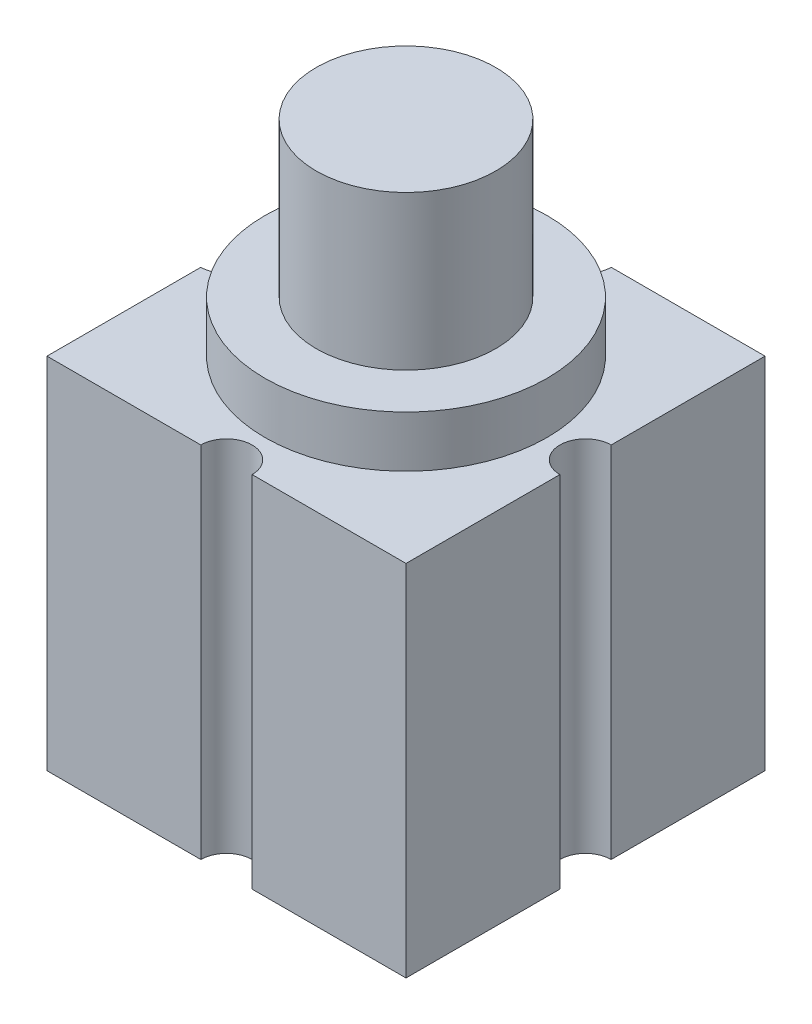
from build123d import *

# Parameters (mm, degrees)
BOSS_EXTRUDE1_DEPTH = 70
SKETCH2_R           = 20
CUT_EXTRUDE1_DEPTH  = 10
SKETCH3_R           = 27.5
BOSS_EXTRUDE2_DEPTH = 10
SKETCH4_R           = 17.5
BOSS_EXTRUDE3_DEPTH = 30


with BuildPart() as part:
    # Sketch1 → Boss-Extrude1 (new body)
    with BuildSketch(Plane(origin=(0, 0, 0), x_dir=(1, 0, 0), z_dir=(0, 1, 0))):
        with BuildLine():
            Line((5, 35), (35, 35))
            Line((35, 35), (35, 5))
            ThreePointArc((35, 5), (30, 0), (35, -5))
            Line((35, -5), (35, -35))
            Line((35, -35), (5, -35))
            ThreePointArc((5, -35), (0, -30), (-5, -35))
            Line((-5, -35), (-35, -35))
            Line((-35, -35), (-35, -5))
            ThreePointArc((-35, -5), (-30, 0), (-35, 5))
            Line((-35, 5), (-35, 35))
            Line((-35, 35), (-5, 35))
            ThreePointArc((-5, 35), (0, 30), (5, 35))
        make_face()
    extrude(amount=BOSS_EXTRUDE1_DEPTH)

    # Sketch2 → Cut-Extrude1 (cut)
    with BuildSketch(Plane.XZ):
        with Locations(Location((0, 0, 0), (0, 0, 270))):
            Circle(SKETCH2_R)
    extrude(amount=-CUT_EXTRUDE1_DEPTH, mode=Mode.SUBTRACT)

    # Sketch3 → Boss-Extrude2 (add)
    with BuildSketch(Plane(origin=(0, 70, 0), x_dir=(1, 0, 0), z_dir=(0, 1, 0))):
        with Locations(Location((0, 0, 0), (0, 0, 270))):
            Circle(SKETCH3_R)
    extrude(amount=BOSS_EXTRUDE2_DEPTH)

    # Sketch4 → Boss-Extrude3 (add)
    with BuildSketch(Plane(origin=(0, 80, 0), x_dir=(1, 0, 0), z_dir=(0, 1, 0))):
        with Locations(Location((0, 0, 0), (0, 0, 270))):
            Circle(SKETCH4_R)
    extrude(amount=BOSS_EXTRUDE3_DEPTH)


solid = part.part
